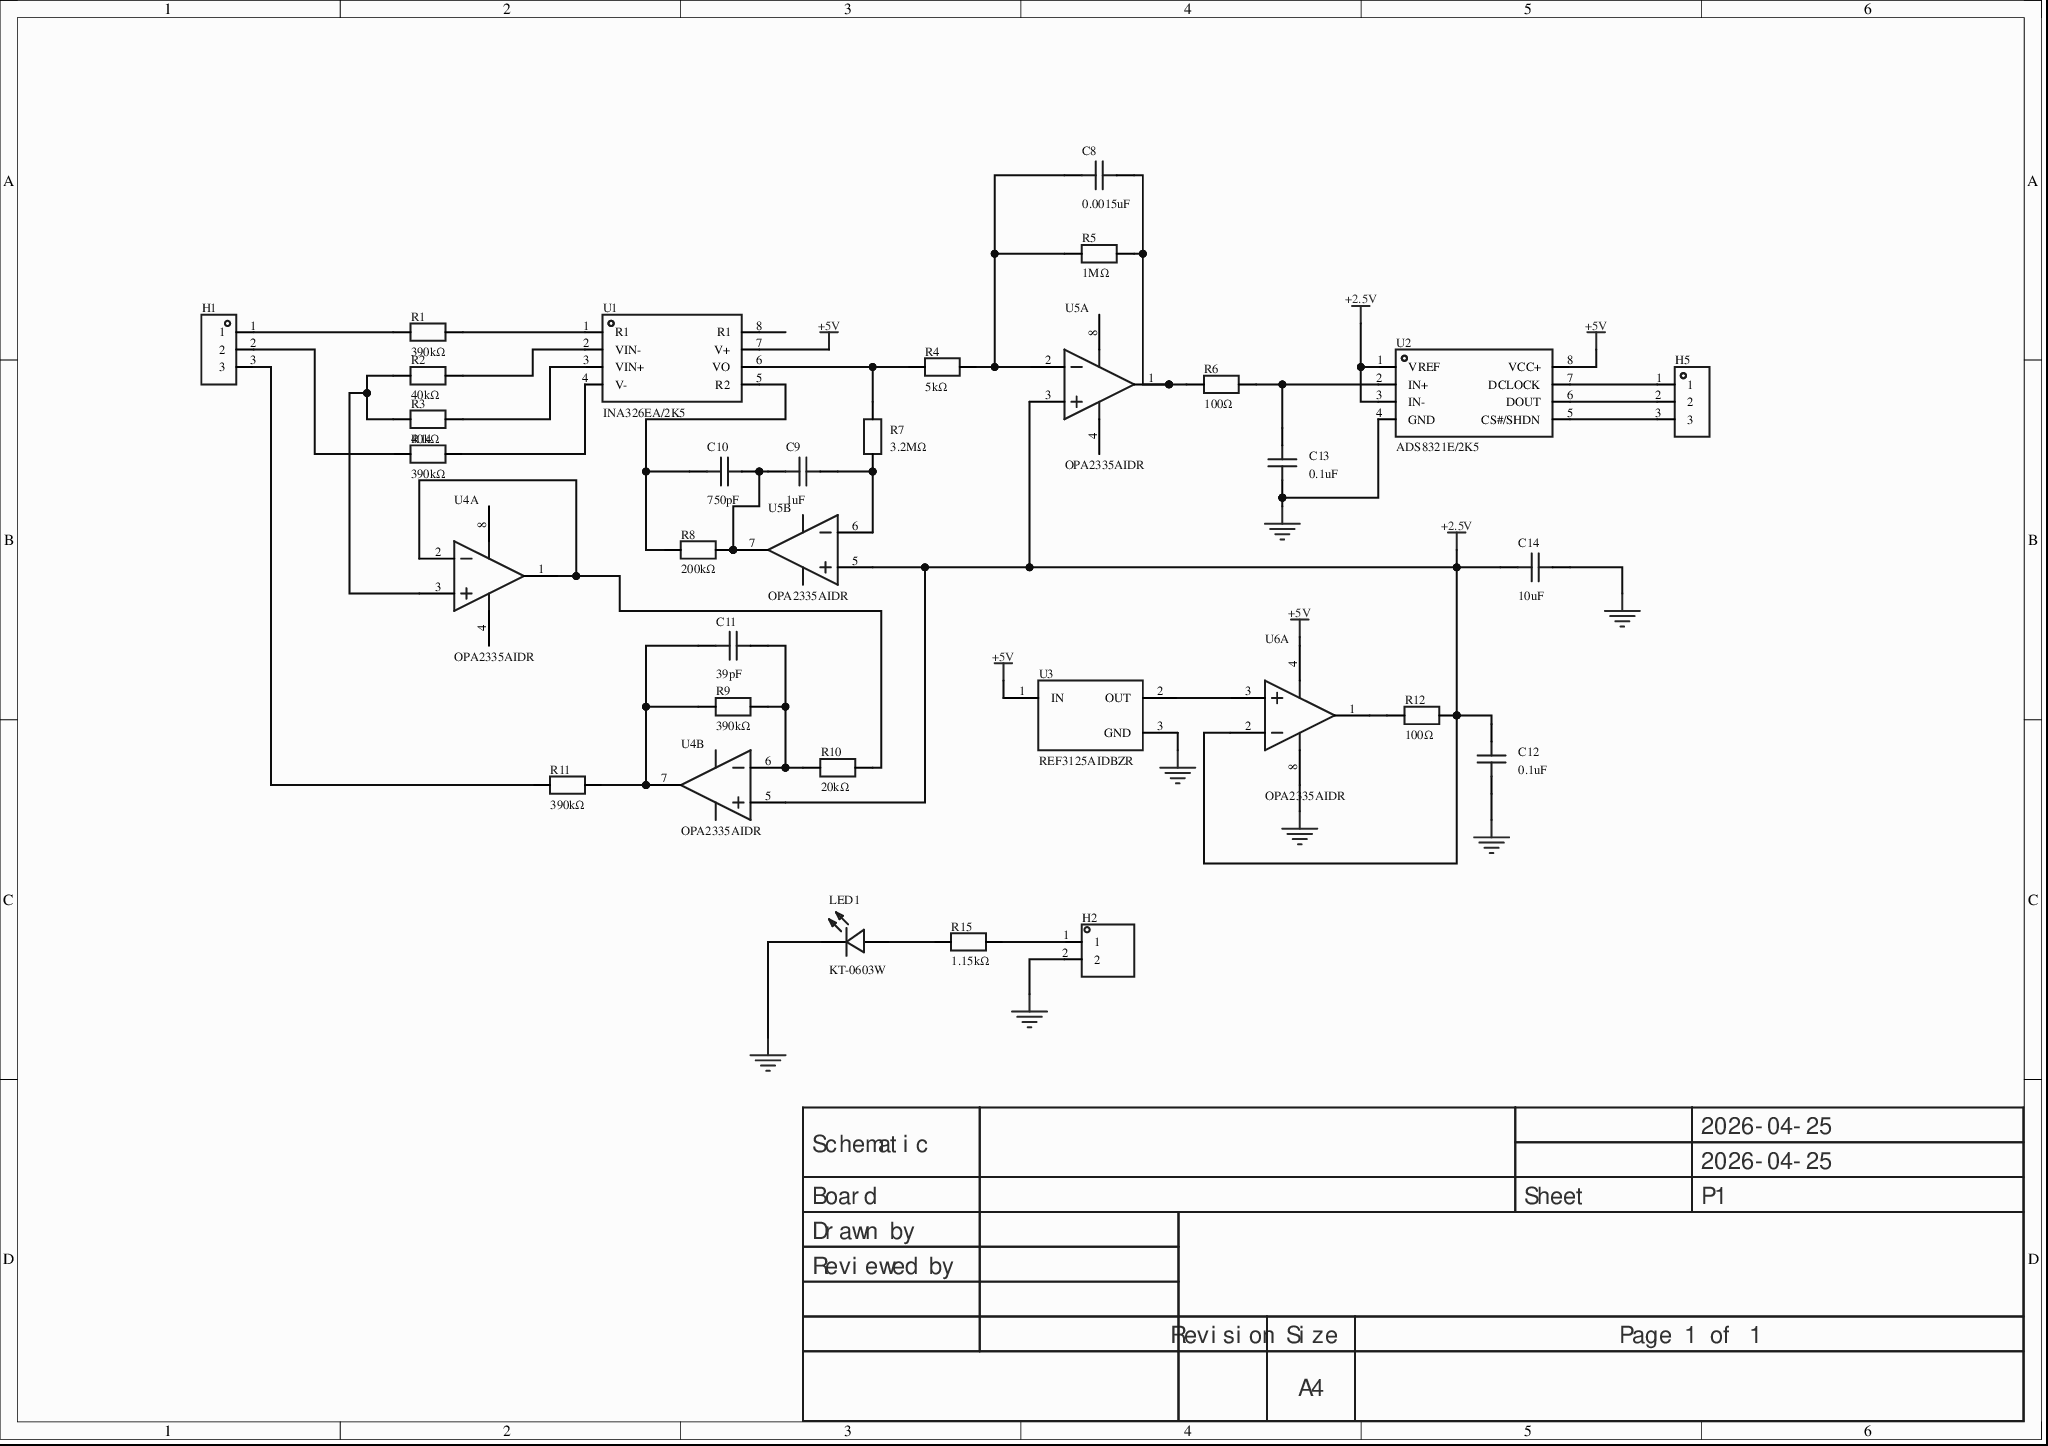
[diagram p0: MISC52015-3.schdoc]
# Altium project MISC52015-2.PrjPcb
1 sheet, 31 parts. Net scope: global (net labels, ports and power ports of the same name join across sheets).
Board file: MISC52015.pcbdoc

## Sheet MISC52015-3.schdoc
size 297 x 209 mm; Version: V1.0; @Project Name: MISC52015; @Update Date: 2026-04-25; @Create Date: 2026-04-25; @Board Name: MISC52015; @Create Time: 10:49:13; @Page Count: 1; @Page No: 1; @Schematic Name: MISC52015; @Update Time: 10:49:13; Size: A4

### Parts
C8  0.0015uF  [C0402]
C9  1uF  [C0402]
C10  750pF  [C0402]
C11  39pF  [C0402]
C12  0.1uF  [C0402]
C13  0.1uF  [C0402]
C14  10uF  [C0402]
H1  (no value)  [HDR-TH_3P-P2.54-V-M]
H2  (no value)  [HDR-TH_2P-P2.54-V-M-1]
H5  (no value)  [HDR-TH_3P-P2.54-V-M]
LED1  KT-0603W  [LED0603-R-RD_WHITE]
R1  390kΩ  [R1206]
R2  40kΩ  [R1206]
R3  40kΩ  [R1206]
R4  5kΩ  [R1206]
R5  1MΩ  [R1206]
R6  100Ω  [R1206]
R7  3.2MΩ  [R1206]
R8  200kΩ  [R1206]
R9  390kΩ  [R1206]
R10  20kΩ  [R1206]
R11  390kΩ  [R1206]
R12  100Ω  [R1206]
R14  390kΩ  [R0402]
R15  1.15kΩ  [R0402]
U1  INA326EA/2K5  [VSSOP-8_L3.0-W3.0-P0.65-LS5.0-BL]
U2  ADS8321E/2K5  [MSOP-8_L3.0-W3.0-P0.65-LS4.9-BL]
U3  REF3125AIDBZR  [SOT-23-3_L2.9-W1.6-P1.90-LS2.8-BR]
U4  OPA2335AIDR  [SOIC-8_L5.0-W4.0-P1.27-LS6.0-BL]  (parts A,B of 2)
U5  OPA2335AIDR  [SOIC-8_L5.0-W4.0-P1.27-LS6.0-BL]  (parts A,B of 2)
U6  OPA2335AIDR  [SOIC-8_L5.0-W4.0-P1.27-LS6.0-BL]  (part A of 2)

### Nets
+2.5V: C12.2 C14.1 R12.2 U2.1(VREF) U2.3(IN-) U4.5(IN_B+) U5.3(IN_A+) U5.5(IN_B+) U6.2(IN_A-)
+5V: U1.7(V+) U2.8(VCC+) U3.1(IN) U6.4(V-)
GND: C12.1 C13.1 C14.2 H2.2 LED1.2(K) U2.4(GND) U3.3(GND) U6.8(V+)
NetC8_1: C8.1 R4.2 R5.1 U5.2(IN_A-)
NetC8_2: C8.2 R5.2 R6.1 U5.1(OUT_A)
NetC9_1: C9.1 C10.2 R8.2 U5.7(OUT_B)
NetC9_2: C9.2 R7.1 U5.6(IN_B-)
NetC10_1: C10.1 R8.1 U1.5(R2)
NetC11_1: C11.1 R9.1 R11.2 U4.7(OUT_B)
NetC11_2: C11.2 R9.2 R10.1 U4.6(IN_B-)
NetC13_2: C13.2 R6.2 U2.2(IN+)
NetH1_1: H1.1 R1.1
NetH1_2: H1.2 R14.1
NetH1_3: H1.3 R11.1
NetH2_1: H2.1 R15.2
NetH5_1: H5.1 U2.7(DCLOCK)
NetH5_2: H5.2 U2.6(DOUT)
NetH5_3: H5.3 U2.5(CS#/SHDN)
NetLED1_1: LED1.1(A) R15.1
NetR1_2: R1.2 U1.1(R1)
NetR2_1: R2.1 R3.1 U4.3(IN_A+)
NetR2_2: R2.2 U1.2(VIN-)
NetR3_2: R3.2 U1.3(VIN+)
NetR4_1: R4.1 R7.2 U1.6(VO)
NetR10_2: R10.2 U4.1(OUT_A) U4.2(IN_A-)
NetR12_1: R12.1 U6.1(OUT_A)
NetR14_2: R14.2 U1.4(V-)
NetU3_2: U3.2(OUT) U6.3(IN_A+)

Not connected (* = marked no-connect by the designer): U1 8(R1); U4 4(V-) 8(V+); U5 4(V-) 8(V+)

### Notes on the sheet
- 2026-04-25
- Schematic
- Board
- Sheet
- P1
- Drawn by
- Reviewed by
- Revision
- Size
- A4
- Page 1 of 1

### Library data of the parts
C8-C14 = GRM158D70E226ME15D: Capacitance: 22uF; Tolerance: ±20%; Rated voltage: 2.5V; Temperature coefficient: X7T;; Manufacturer: muRata(村田); AddInBom: yes; ModelId: 36a51122f27c49738f86b3bfa98863e00819f05c4eef4c71ace90d822a990e87; ModelName: C0402_L1.0-W0.5-H0.5; ModelTransform: 39.37,19.685,0,0,0,0,0,0,0; Symbol: GRM158D70E226ME15D; Device: GRM158D70E226ME15D; LCSC Part Name: 22uF ±20% 2.5V; ManufacturerPart: GRM158D70E226ME15D; Supplier Footprint: 0402; JLCPCB Part Class: Extended Part; Datasheet: https://example.com/datasheet/GRM158D70E226ME15D/51841209.html; Supplier: LCSC; ConvertToPcb: yes; FootprintName: C0402; Voltage Rating: 2.5V; Temperature Coefficient: X7T
  C8: Value: 0.0015uF
  C9: Value: 1uF
  C10: Value: 750pF
  C11: Value: 39pF
  C12 C13: Value: 0.1uF
  C14: Value: 10uF
H1 H5 = HDR-M_2.54_1x3P: AddInBom: yes; ModelId: bb473b6d38ff42a99216a4fcdbdcc4cb0819f05c4eef4c71ace90d822a990e87; ModelName: HDR-TH_3P-P2.54-M-LI-1X3P; ModelTransform: 300.03877,100,0,0,0,0,0,0,-118.11; Symbol: HDR-M_2.54_1x3P; Device: HDR-M_2.54_1x3P; ConvertToPcb: yes; FootprintName: HDR-TH_3P-P2.54-V-M; SupplierPart: C2937625; Supplier Footprint: 插件
H2 = HDR-M_2.54_1x2P: Symbol: 210S-1*2P L=11.6MMGold-plated black; ConvertToPcb: yes; ModelId: 79b2e9f2d70a4d68a1b7098f27c6d4c50819f05c4eef4c71ace90d822a990e87; ModelName: HDR-M-2.54_1x2; ModelTransform: 200,100,0,0,0,0,0,0,-118.11; Device: HDR-M_2.54_1x2P; AddInBom: yes; SupplierPart: C124375; Supplier Footprint: 插件; FootprintName: HDR-TH_2P-P2.54-V-M-1
LED1 = KT-0603W: 灯头类型:-;发光颜色:白色;正向压降(Vf):2.6V~3.1V;功率:100mW;正向电流:5mA;波长:-;二极管配置:独立二极管;透镜颜色:黄色透镜;色温:-;发光强度:360mcd;发光角度:120°;载带方式:正贴;工作温度:-40℃~+85℃;; Manufacturer: KENTO; Symbol: 0603White light_C2290; AddInBom: yes; ModelId: 69daf87d236b4f268260e1d4a354a21e0819f05c4eef4c71ace90d822a990e87; ModelTransform: 63.7794,31.496,0,0,0,0,0,0,0; Illumination Color: White; Power(Watts): 100mW; Forward Current: 5mA; Diode Configuration: Single diode; Lens Color: Yellow lens; Luminous Intensity: 360mcd; Viewing Angle: 120°; Device: KT-0603W; LCSC Part Name: 0603 白灯 高亮; SupplierPart: C2290; ManufacturerPart: KT-0603W; Supplier Footprint: 0603; JLCPCB Part Class: Basic Part; Datasheet: https://example.com/datasheet/KT-0603W/2663.html; Supplier: LCSC; ConvertToPcb: yes; FootprintName: LED0603-R-RD_WHITE; ModelName: LED0603-R-RD_WHITE; Lamp Holder Type: -; Voltage - Forward(Vf): 2.6V~3.1V; Wavelength - Dominant: -; Peak Wavelength: -; Color Temperature: -; Mounting Style: Top mount; Operating Temperature: -40℃~+85℃
R1-R12 = RE1206F1R000: Resistor type: sampling resistor; alloy resistor; Resistance: 0Ω; Tolerance: ±1%; Power: 1W; Mounting: SMD;; Manufacturer: JIERR(捷而瑞); AddInBom: yes; ModelId: 89a1f13db2384da588040e0b3c55bf660819f05c4eef4c71ace90d822a990e87; ModelName: R1206_L3.2-W1.6-H0.6; ModelTransform: 125.984,62.992,0,0,0,0,0,0,0; Symbol: RE1206F1R000; Device: RE1206F1R000; LCSC Part Name: 0mΩ 1W 1206 ±1%; ManufacturerPart: RE1206F1R000; Supplier Footprint: 1206; JLCPCB Part Class: Extended Part; Datasheet: https://example.com/datasheet/RE1206F1R000/49133304.html; Supplier: LCSC; ConvertToPcb: yes; FootprintName: R1206; Type: Sampling resistor; alloy resistor; Power(Watts): 1W; Mounting Type: SMD
  R1 R9 R11: Value: 390kΩ
  R2 R3: Value: 40kΩ
  R4: Value: 5kΩ
  R5: Value: 1MΩ
  R6 R12: Value: 100Ω
  R7: Value: 3.2MΩ
  R8: Value: 200kΩ
  R10: Value: 20kΩ
R14 R15 = GR0402F1K15TAG00: Resistor type: thick film resistor; Resistance: 1.15kΩ; Tolerance: ±1%; Power: 62.5mW; Operating voltage: 50V;; Manufacturer: GiantOhm(鼎声微电); AddInBom: yes; ModelId: 98c88bc2b9094f218f3a3e30a70127380819f05c4eef4c71ace90d822a990e87; ModelName: R0402_L1.0-W0.5-H0.4; ModelTransform: 39.37,19.685,0,0,0,0,0,0,0; Symbol: GR0402F1K15TAG00; Device: GR0402F1K15TAG00; LCSC Part Name: 1K15 ±1%; ManufacturerPart: GR0402F1K15TAG00; Supplier Footprint: 0402; JLCPCB Part Class: Extended Part; Datasheet: https://example.com/datasheet/GR0402F1K15TAG00/52211426.html; Supplier: LCSC; ConvertToPcb: yes; FootprintName: R0402; Type: Thick film resistor; Power(Watts): 62.5mW; Voltage-Supply(Max): 50V; Operating Temperature: -55℃~+155℃
  R14: Value: 390kΩ
  R15: SupplierPart: C49653840; Value: 1.15kΩ
U1 = INA326EA/2K5: 放大器数:单路;共模抑制比(CMRR):114dB;输入偏置电流(Ib):200pA;输入失调电压(Vos):20uV;增益带宽积(GBP):-;压摆率(SR):-;轨到轨:轨到轨输入,轨到轨输出;; Manufacturer: TI(德州仪器); AddInBom: yes; ModelId: fe8ada2663e64b00b932016623def7030819f05c4eef4c71ace90d822a990e87; ModelName: VSSOP-8_L3.0-W3.0-H1.1-LS4.9-P0.65; ModelTransform: 197.34433,118.11,0,90,0,0,0,0.0005,0; Number of Channels: Single; Common Mode Rejection Ratio(CMRR): 114dB; Ib - Input Bias Current: 200pA; Vos - Input Offset Voltage: 20uV; Output Current: 25mA; Rail to Rail: Rail-to-rail input, rail-to-rail output; Quiescent Current(Iq): 2.4mA; Input Offset Voltage Drift(Vos TC): 100nV/℃; Maximum Power Supply Range (Vdd-Vss): 5.5V; Noise density(eN): 33nV/√Hz@1kHz; Single Supply: 2.7V~5.5V; Settling time: 950us; Symbol: INA326EA/2K5; Device: INA326EA/2K5; LCSC Part Name: 精密、轨到轨输入输出仪表放大器; SupplierPart: C179740; ManufacturerPart: INA326EA/2K5; Supplier Footprint: VSSOP-8; JLCPCB Part Class: Extended Part; Supplier: LCSC; ConvertToPcb: yes; FootprintName: VSSOP-8_L3.0-W3.0-P0.65-LS5.0-BL; Gain Bandwidth Product: -; Slew Rate: -; Output Type: -; Operating Temperature: -40℃~+85℃; Input Offset Current(Ios): 200pA
U2 = ADS8321E/2K5: Resolution (bit): 16; Sample rate: 100kHz; Operating voltage: 4.75V~5.25V; Interface type: SPI;; Manufacturer: TI(德州仪器); AddInBom: yes; ModelId: bedc0aeebe0a475e87aaac88bd02a14b0819f05c4eef4c71ace90d822a990e87; ModelName: MSOP-8_L3.0-W3.0-H1.1-LS4.9-P0.65; ModelTransform: 118.11,192.913,0,0,0,0,0,0,0; Resolution(Bits): 16; Signal-to-Noise Ratio: 85dB; Clock/Oscillator: External; Clock Frequency: 24kHz~2.9MHz; Programmable Gain: Not supported; ADC architecture: SAR; Quiescent Current (Iq): 3uA; Symbol: ADS8321E/2K5; Device: ADS8321E/2K5; LCSC Part Name: 16位，高速，微功耗采样模拟到数字转换器; SupplierPart: C544489; ManufacturerPart: ADS8321E/2K5; Supplier Footprint: VSSOP-8; JLCPCB Part Class: Extended Part; Supplier: LCSC; ConvertToPcb: yes; FootprintName: MSOP-8_L3.0-W3.0-P0.65-LS4.9-BL; Sampling Rate: 100kHz; number of channels: -; Voltage - Supply: 4.75V~5.25V; Interface: SPI; differential input: Yes; Integral non - linearity: -; Operating Temperature: -40℃~+85℃; Voltage Reference: External; Voltage Reference Drift: -; Temperature Sensors: -; Data rate: -; Full-Scale Range(FSR): -
U3 = REF3125AIDBZR: Output type: Fixed; Operating voltage: 2.55V~5.5V; Output voltage: 2.5V; Output current: 10mA; Accuracy: ±0.2%;; Manufacturer: TI(德州仪器); AddInBom: yes; ModelId: 89cb27a44ab2466697082bb9fd73a7d00819f05c4eef4c71ace90d822a990e87; ModelName: SOT-23-3L_L2.9-W1.6-H1.1-LS2.8-P0.95; ModelTransform: 114.173,110.236,0,90,0,0,0,0,0; Temperature Coefficient: 20ppm/℃; Reference Type: Series; Quiescent Current: 135uA; Noise - 1/10Hz to 10Hz: 33uVp-p; Noise - 10Hz to 10kHz: 48uVrms; Symbol: REF3125AIDBZR; Device: REF3125AIDBZR; LCSC Part Name: 2.55V~5.5V 串联 135uA 20ppm/℃; SupplierPart: C33297; ManufacturerPart: REF3125AIDBZR; Supplier Footprint: SOT-23; JLCPCB Part Class: Extended Part; Supplier: LCSC; ConvertToPcb: yes; FootprintName: SOT-23-3_L2.9-W1.6-P1.90-LS2.8-BR; Output Type: Fixed; Voltage - Supply: 2.55V~5.5V; Output Voltage: 2.5V; Output Current: 10mA; Tolerance: ±0.2%; Minimum Cathode Current for Regulation: -; Operating Temperature: -40℃~+125℃
U4-U6 = OPA2335AIDR: Amplifier count: Dual; Gain bandwidth product (GBP): 2MHz; Input bias current (Ib): 70pA; Input offset voltage (Vos): 1uV; Slew rate (SR): 1.6V/us; Bandwidth (-3dB): -; Rail-to-rail: -;; Manufacturer: TI(德州仪器); Relevance: []; AddInBom: yes; ModelId: 7abc64c95a1a4a04a4ef38f9097c870b0819f05c4eef4c71ace90d822a990e87; ModelTransform: 192.913,236.22,0,0,0,0,0,0,0; Quiescent Current per Amplifier: 570uA; Symbol: OPA2335AIDR; Device: OPA2335AIDR; LCSC Part Name: OPA2335AIDR; SupplierPart: C41618; ManufacturerPart: OPA2335AIDR; Supplier Footprint: SOIC-8; JLCPCB Part Class: Extended Part; Supplier: LCSC; ConvertToPcb: yes; FootprintName: SOIC-8_L5.0-W4.0-P1.27-LS6.0-BL; ModelName: SOIC-8_L5.0-W4.0-P1.27-LS6.0-BL; Number of Channels: Dual; Gain Bandwidth Product: 2MHz; Ib - Input Bias Current: 70pA; Vos - Input Offset Voltage: 1uV; Slew Rate: 1.6V/us; -3dB Bandwidth: -; Output Type: -; Rail to Rail: -; Operating Temperature: -40℃~+125℃